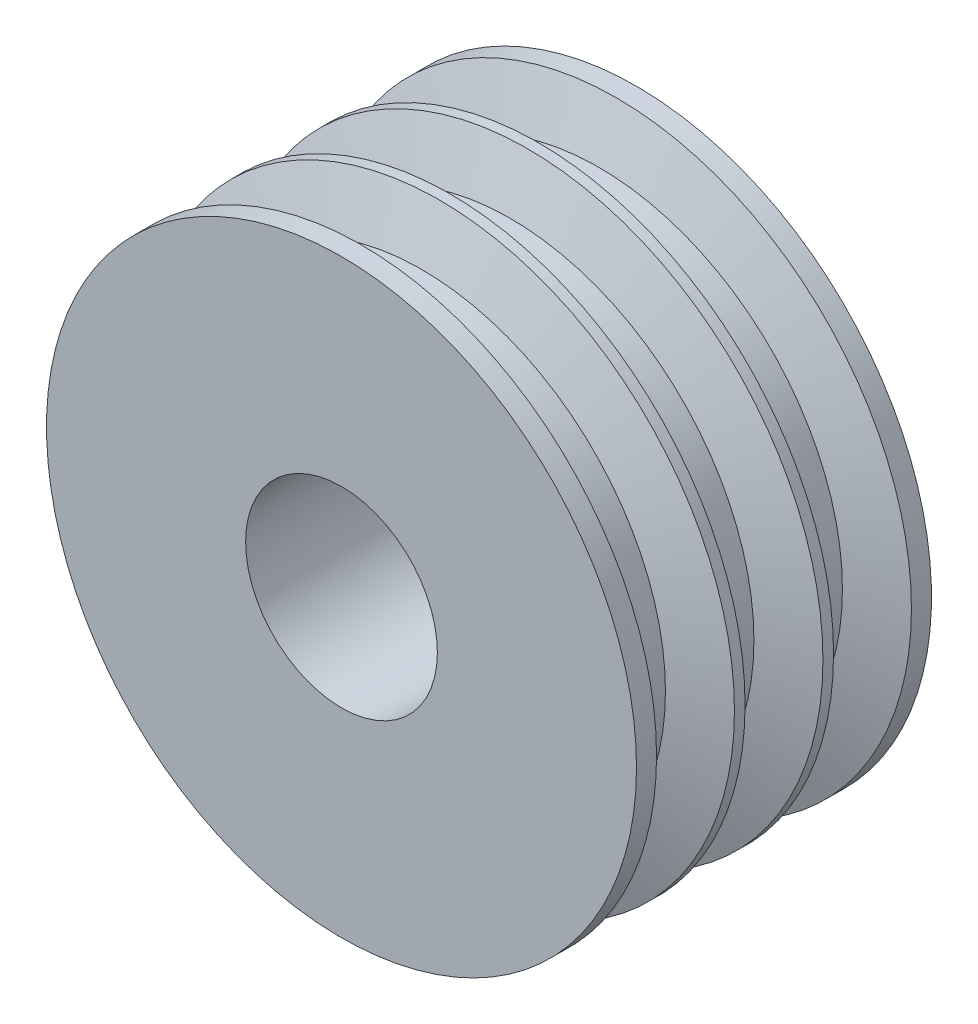
SolidWorks part; units mm, degrees
ref_plane "Front Plane" through (0, 0, 0) normal (0, 0, 1) x (1, 0, 0)
ref_plane "Top Plane" through (0, 0, 0) normal (0, 1, 0) x (1, 0, 0)
ref_plane "Right Plane" through (0, 0, 0) normal (1, 0, 0) x (0, 0, -1)
sketch "Sketch1" plane through (0, 0, 0) normal (0, 0, 1) x (1, 0, 0)
  circle A0 centre (0, 0) radius 50
  dimension "D1" = 100
extrude "Boss-Extrude1" add sketch "Sketch1" along normal mid plane 80
sketch "Sketch2" plane through (0, 0, 40) normal (0, 0, 1) x (1, 0, 0)
  circle A0 centre (0, 0) radius 16.25
  dimension "D1" = 32.5
extrude "Cut-Extrude1" cut sketch "Sketch2" against normal blind 150
sketch "Sketch4" plane through (0, 0, 0) normal (1, 0, 0) x (0, 0, -1)
  line L0 (-40, 50) -> (-40, -50) construction
  line L1 (-40, 50) -> (-40, -50) construction
  line L2 (-40, 50) -> (-40, -50) construction
  line L3 (-40, 50) -> (-36.6, 50)
  line L4 (-36.6, 50) -> (-33.6043, 41.3)
  line L5 (-21.6, 50) -> (-18.6043, 41.3)
  line L6 (-30, 41.3) -> (-30, 134.1405) construction
  line L7 (-33.6043, 41.3) -> (-26.3957, 41.3)
  line L8 (-23.4, 50) -> (-26.3957, 41.3)
  line L15 (-23.4, 50) -> (-21.6, 50)
  line L19 (10, 161.0505) -> (-40, 161.0505)
  line L20 (-40, 161.0505) -> (-40, 50)
  line L21 (0, 0) -> (121.1492, 0) construction
  line L22 (-18.6043, 41.3) -> (-11.3957, 41.3)
  line L23 (-8.4, 50) -> (-11.3957, 41.3)
  line L24 (-8.4, 50) -> (-6.6, 50)
  line L25 (-6.6, 50) -> (-3.6043, 41.3)
  line L26 (-3.6043, 41.3) -> (3.6043, 41.3)
  line L27 (6.6, 50) -> (3.6043, 41.3)
  line L32 (0, 41.3) -> (0, 132.7741) construction
  line L36 (6.6, 50) -> (10, 50)
  line L39 (21.6, 50) -> (23.4, 50) [skipped]
  line L40 (38.6, 50) -> (90.6382, 50) [skipped]
  line L41 (11.3957, 41.3) -> (18.6043, 41.3) [skipped]
  line L42 (21.6, 50) -> (18.6043, 41.3) [skipped]
  line L43 (23.4, 50) -> (26.3957, 41.3) [skipped]
  line L44 (26.3957, 41.3) -> (33.6043, 41.3) [skipped]
  line L45 (36.6, 50) -> (33.6043, 41.3) [skipped]
  line L46 (8.4, 50) -> (11.3957, 41.3) [skipped]
  line L47 (6.6, 50) -> (8.4, 50) [skipped]
  line L48 (40, 50) -> (-40, 50) construction
  line L49 (10, 50) -> (10, 161.0505)
  dimension "D1" = 10
  dimension "D2" = 8.7
  dimension "D3" = 6.6
  dimension "D4" = 19
  dimension "D5" = 5
  dimension "D6" = 10
revolve "Cut-Revolve1" cut sketch "Sketch4" angle 360 about L21
sketch "Sketch7" plane through (0, 0, 40) normal (0, 0, 1) x (1, 0, 0)
  line L0 (0, 0) -> (0, 137.7007) construction
  line L1 (0, 0) -> (-81.6728, 81.6728) construction
  circle A1 centre (0, 0) radius 22.8 construction
  circle A2 centre (-53.033, 53.033) radius 20
  circle A3 centre (53.033, 53.033) radius 20
  circle A4 centre (53.033, -53.033) radius 20
  circle A5 centre (-53.033, -53.033) radius 20
  point P16 (0, 0)
  dimension "D1" = 45.6
  dimension "D3" = 40
  dimension "D4" = 75
  dimension "D2" = 45
  dimension "D5" = 4
sketch "Sketch10" plane through (0, 0, -40) normal (0, 0, -1) x (-1, 0, 0)
  circle A4 centre (0, 0) radius 100
  dimension "D1" = 200
extrude "Cut-Extrude5" cut sketch "Sketch10" against normal blind 20
sketch "Sketch11" plane through (0, 0, -20) normal (0, 0, -1) x (-1, 0, 0)
  circle A0 centre (0, 0) radius 30
  circle A3 centre (0, 0) radius 16.25
  circle A4 centre (0, 0) radius 16.25
  dimension "D2" = 60
  dimension "D1" = 0
extrude "Boss-Extrude2" add sketch "Sketch11" along normal blind 20
extrude "Cut-Extrude6" [suppressed] cut sketch "Sketch7" against normal blind 150
sketch "Sketch12" plane through (0, 0, -40) normal (0, 0, -1) x (-1, 0, 0)
  circle A2 centre (0, 0) radius 130
  circle A3 centre (0, 0) radius 130
  dimension "D1" = 100
extrude "Cut-Extrude7" cut sketch "Sketch12" against normal blind 30
sketch "Sketch13" plane through (0, 0, 40) normal (0, 0, 1) x (1, 0, 0)
  circle A0 centre (0, 0) radius 30
  circle A1 centre (0, 0) radius 16.25 construction
  circle A2 centre (0, 0) radius 16.25
  dimension "D1" = 60
extrude "Boss-Extrude3" [suppressed] add sketch "Sketch13" along normal blind 25
